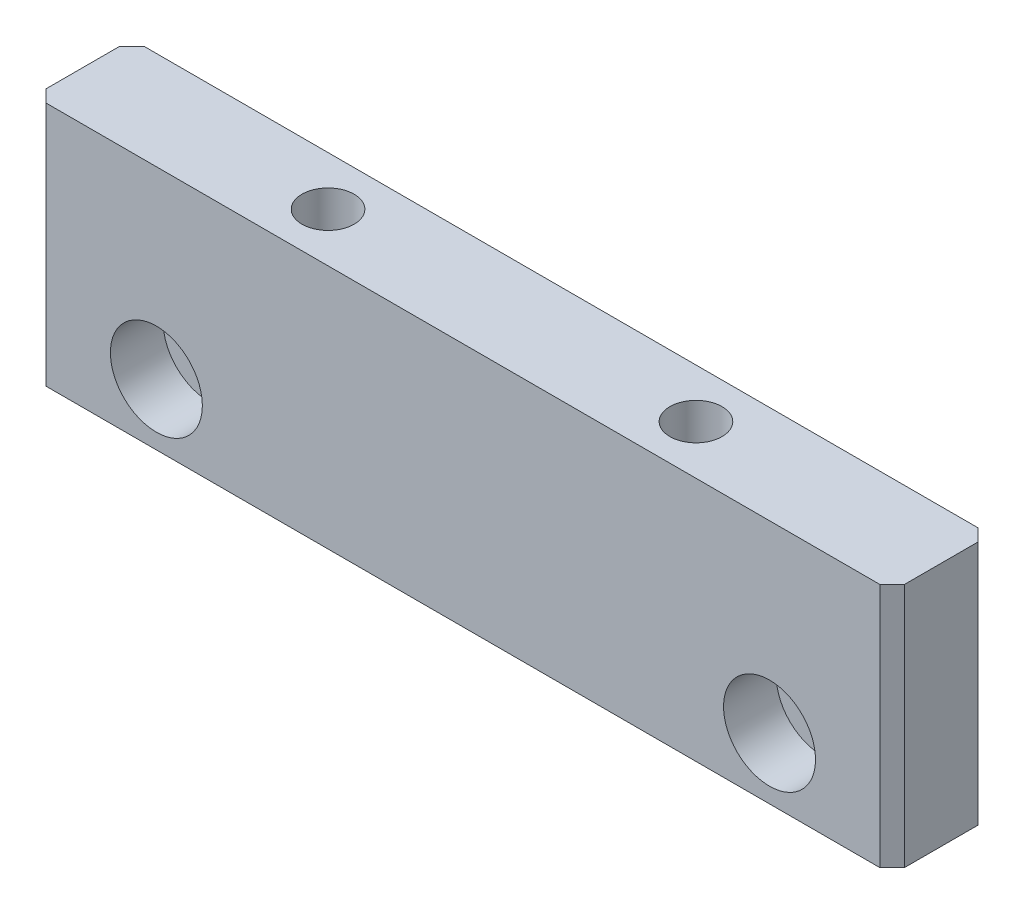
SolidWorks part; units mm, degrees
ref_plane "前视基准面" through (0, 0, 0) normal (0, 0, 1) x (1, 0, 0)
ref_plane "上视基准面" through (0, 0, 0) normal (0, 1, 0) x (1, 0, 0)
ref_plane "右视基准面" through (0, 0, 0) normal (1, 0, 0) x (0, 0, -1)
sketch "草图1" plane through (0, 0, 0) normal (0, 0, 1) x (1, 0, 0)
  line L1 (0, 0) -> (140, 0)
  line L2 (0, 0) -> (0, 40)
  line L3 (0, 40) -> (140, 40)
  line L4 (140, 0) -> (140, 40)
  dimension "D1" = 140
  dimension "D2" = 40
extrude "凸台-拉伸1" add sketch "草图1" along normal blind 16
hole_wizard "M10 螺纹孔1" positions "草图3" profile "草图2" tap size "M10" standard "ISO" end condition through all
sketch "草图3" plane through (0, 40, 0) normal (0, 1, 0) x (1, 0, 0)
  line L0 (0, -8) -> (140, -8) construction
  line L1 (0, -16) -> (0, 0) construction
  line L2 (140, -16) -> (140, 0) construction
  line L4 (70, 0) -> (70, -16) construction
  line L5 (140, 0) -> (0, 0) construction
  line L6 (140, -16) -> (0, -16) construction
  point P0 (40, -8)
  point P2 (100, -8)
  dimension "D1" = 60
sketch "草图2" plane through (40, 40, 8) normal (1, 0, 0) x (0, 0, 1)
  line L0 (0, 0) -> (0, 40)
  line L1 (0, 40) -> (4.25, 40)
  line L2 (4.25, 40) -> (4.25, 0)
  line L5 (4.25, 0) -> (0, 0)
  line L11 (0, -6.35) -> (0, 107.95) construction
  dimension "通孔螺纹孔钻头直径" = 8.5
  dimension "通孔螺纹孔钻头深度" = 40
cosmetic thread "孔螺蚊线1" parameters "D2"=10
cosmetic thread "孔螺蚊线2" parameters "D2"=10
hole_wizard "M8 六角凹头螺钉的柱形沉头孔1" positions "草图6" profile "草图5" counterbore size "M8" standard "ISO" end condition through all
sketch "草图6" plane through (0, 0, 16) normal (0, 0, 1) x (1, 0, 0)
  line L0 (20, -3.3841) -> (20, 43.6498) construction
  line L1 (0, 0) -> (140, 0) construction
  line L2 (70, 0) -> (70, 48.7891) construction
  point P0 (20, 10)
  point P18 (120, 10)
  dimension "D1" = 10
  dimension "D2" = 100
sketch "草图5" plane through (20, 10, 16) normal (1, 0, 0) x (0, -1, 0)
  line L0 (0, 0) -> (0, 16)
  line L1 (0, 16) -> (4.2, 16)
  line L3 (4.2, 16) -> (4.2, 8.6)
  line L4 (4.2, 8.6) -> (7.5, 8.6)
  line L5 (7.5, 8.6) -> (7.5, 0)
  line L7 (7.5, 0) -> (0, 0)
  line L11 (0, -6.35) -> (0, 107.95) construction
  dimension "通孔孔直径" = 8.4
  dimension "通孔孔深度" = 16
  dimension "柱形沉头孔直径" = 15
  dimension "柱形沉头孔深度" = 8.6
chamfer "倒角1" distance 2 angle 45 4 edges at (140, 20, 16) (0, 20, 16) (0, 20, 0) (140, 20, 0)
